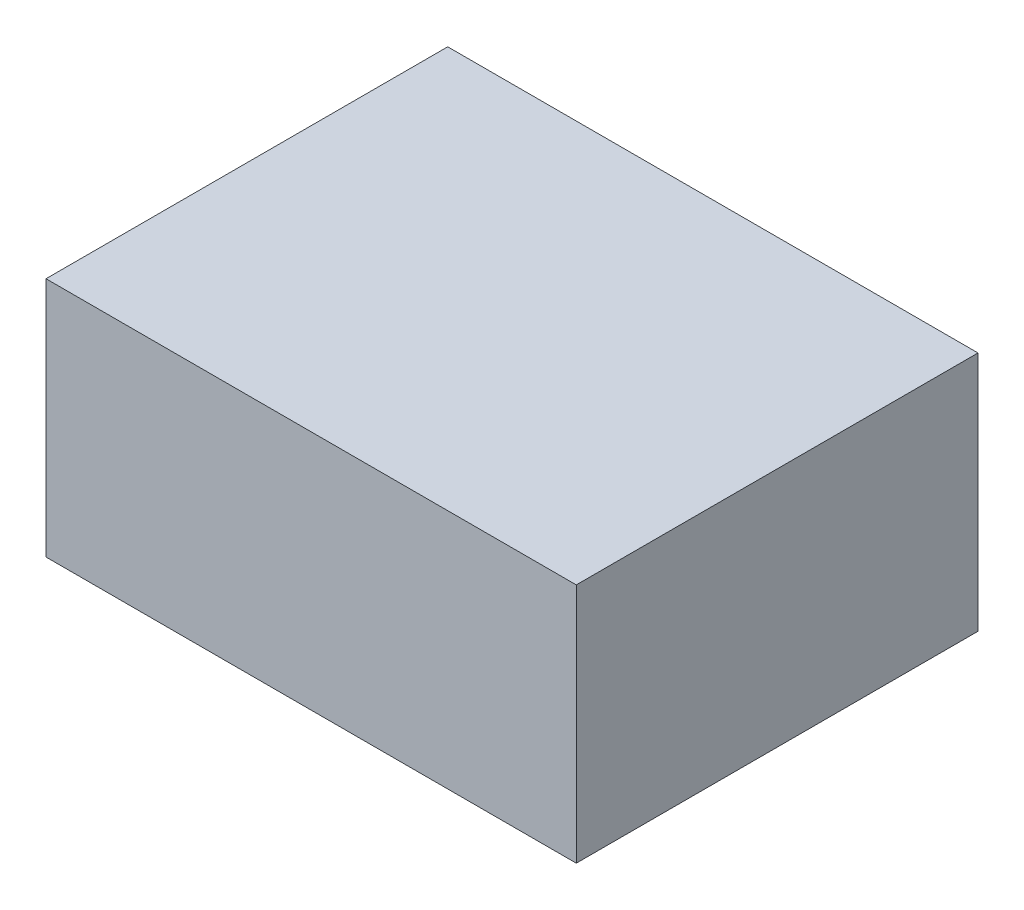
SolidWorks part; units mm, degrees
ref_plane "前视基准面" through (0, 0, 0) normal (0, 0, 1) x (1, 0, 0)
ref_plane "上视基准面" through (0, 0, 0) normal (0, 1, 0) x (1, 0, 0)
ref_plane "右视基准面" through (0, 0, 0) normal (1, 0, 0) x (0, 0, -1)
sketch "草图1" plane through (0, 0, 0) normal (0, 0, 1) x (1, 0, 0)
  line L1 (-1004.9044, 2718.9148) -> (-344.9044, 2718.9148)
  line L2 (-1004.9044, 2718.9148) -> (-1004.9044, 3018.9148)
  line L3 (-1004.9044, 3018.9148) -> (-344.9044, 3018.9148)
  line L4 (-344.9044, 2718.9148) -> (-344.9044, 3018.9148)
  dimension "D1" = 660
  dimension "D2" = 300
extrude "凸台-拉伸1" add sketch "草图1" along normal blind 500
shell "抽壳1" thickness 10
